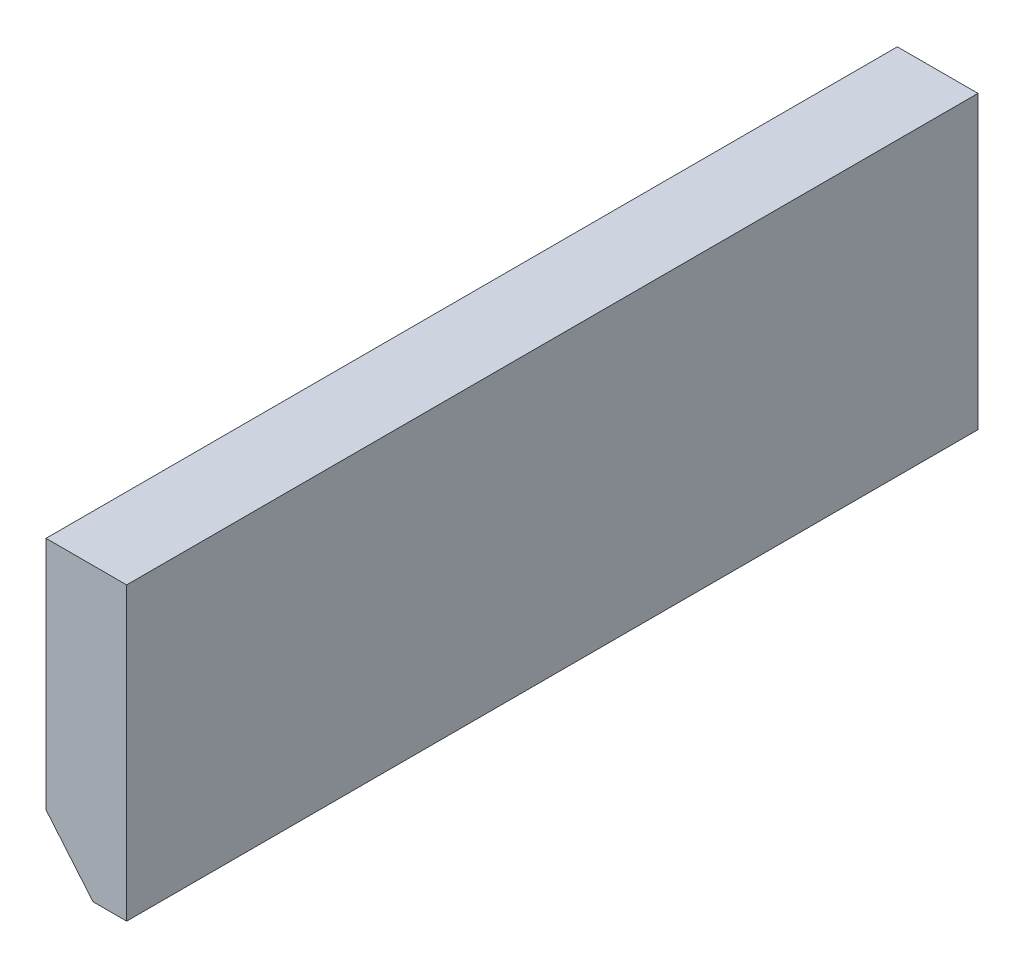
SolidWorks part; units mm, degrees
material "普通碳钢"
ref_plane "Front Plane" through (0, 0, 0) normal (0, 0, 1) x (1, 0, 0)
ref_plane "Top Plane" through (0, 0, 0) normal (0, 1, 0) x (1, 0, 0)
ref_plane "Right Plane" through (0, 0, 0) normal (1, 0, 0) x (0, 0, -1)
sketch "Sketch1" plane through (0, 0, 0) normal (0, 0, 1) x (1, 0, 0)
  line L0 (0, 0) -> (0, 130)
  line L1 (0, 130) -> (-36, 130)
  line L2 (-36, 130) -> (-36, 25.0268)
  line L3 (-36, 25.0268) -> (-15, 0)
  line L4 (-15, 0) -> (0, 0)
  dimension "D1" = 130
  dimension "D2" = 36
  dimension "D3" = 15
  dimension "D4" = 50
extrude "Boss-Extrude1" add sketch "Sketch1" along normal mid plane 380
